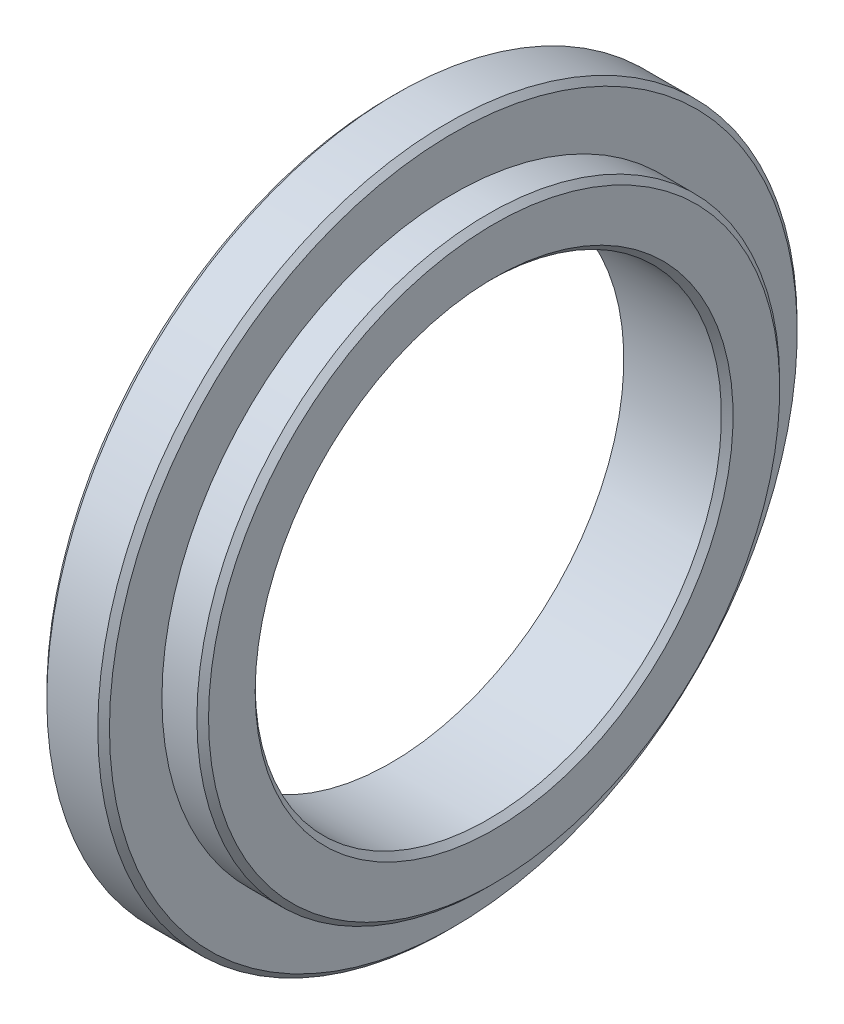
from build123d import *

# Parameters (mm, degrees)
CHAMFER1_SIZE = 1


with BuildPart() as part:
    # Sketch1 → Revolve1 (revolve)
    with BuildSketch(Plane.XY, mode=Mode.PRIVATE) as revolve1_sk:
        Polygon((0, 60), (0, 40), (17.75, 40), (17.75, 50), (10.75, 50), (10.75, 60), align=None)
    revolve(revolve1_sk.sketch.rotate(Axis((0, 0, 0), (1, 0, 0)), 90), axis=Axis((0, 0, 0), (1, 0, 0)))

    # Chamfer1
    chamfer1_edges = [part.edges().sort_by_distance(p)[0] for p in [
        (10.75, 0, -60),
        (17.75, 0, -50),
        (17.75, 0, -40),
        (0, 0, -60),
    ]]
    chamfer(chamfer1_edges, length=CHAMFER1_SIZE)


solid = part.part
